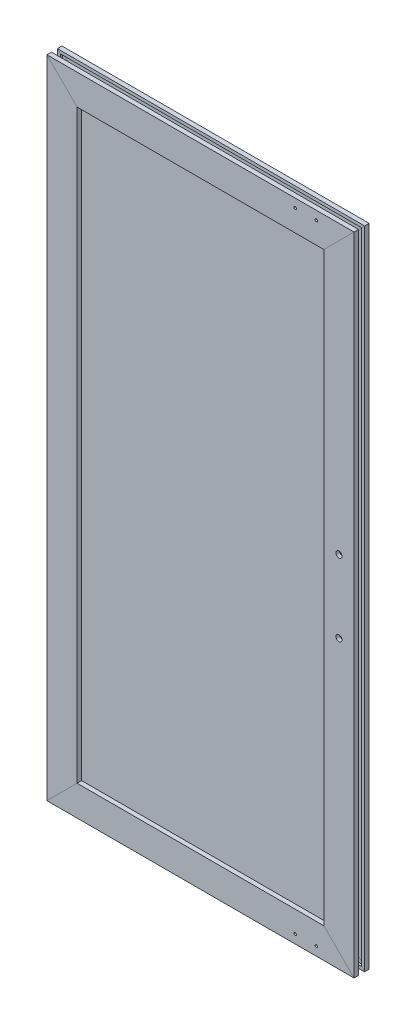
SolidWorks part; units mm, degrees
material "铝型材"
ref_plane "前视基准面" through (0, 0, 0) normal (0, 0, 1) x (1, 0, 0)
ref_plane "上视基准面" through (0, 0, 0) normal (0, 1, 0) x (1, 0, 0)
ref_plane "右视基准面" through (0, 0, 0) normal (1, 0, 0) x (0, 0, -1)
sketch "草图13" plane through (0, 0, 0) normal (0, 0, 1) x (1, 0, 0)
  line L1 (-183.5, -408) -> (183.5, -408)
  line L2 (-183.5, -408) -> (-183.5, 408)
  line L3 (-183.5, 408) -> (183.5, 408)
  line L4 (183.5, -408) -> (183.5, 408)
  line L5 (-183.5, -408) -> (183.5, 408) construction
  line L6 (-183.5, 408) -> (183.5, -408) construction
  point P0 (0, 0)
  dimension "D1" = 367
  dimension "D2" = 816
other "铝型材 2040A(1)"
ref_plane "基准面3" through (-183.5, 408, 0) normal (1, 0, 0) x (0, 1, 0)
sketch "草图19" plane through (-183.5, 408, 0) normal (1, 0, 0) x (0, 1, 0)
  line L0 (9, 4) -> (6, 4)
  line L1 (9, 4) -> (9, 7)
  line L2 (6, -4) -> (6, 4)
  line L3 (16, 7) -> (9, 7)
  line L4 (9, -4) -> (6, -4)
  line L5 (16, 4) -> (16, 7)
  line L6 (9, -7) -> (9, -4)
  line L7 (20, 4) -> (16, 4)
  line L8 (16, -7) -> (9, -7)
  line L9 (20, 10) -> (20, 4)
  line L10 (16, -7) -> (16, -4)
  line L11 (-20, 10) -> (20, 10)
  line L12 (20, -4) -> (16, -4)
  line L13 (-20, 4) -> (-20, 10)
  line L14 (20, -4) -> (20, -10)
  line L15 (-20, 4) -> (-16, 4)
  line L16 (20, -10) -> (-20, -10)
  line L17 (-16, 4) -> (-16, 7)
  line L18 (-20, -10) -> (-20, -4)
  line L19 (-16, 7) -> (-9, 7)
  line L20 (-20, -4) -> (-16, -4)
  line L21 (-9, 4) -> (-9, 7)
  line L22 (-16, -7) -> (-16, -4)
  line L23 (-9, 4) -> (-6, 4)
  line L24 (-16, -7) -> (-9, -7)
  line L25 (-6, -4) -> (-6, 4)
  line L26 (-9, -7) -> (-9, -4)
  line L27 (-9, -4) -> (-6, -4)
  circle A0 centre (0, 0) radius 3.25
  point P0 (0, 0)
sketch "草图14" plane through (0, 0, 0) normal (0, 0, 1) x (1, 0, 0)
  line L0 (189.5, 414) -> (192.5, 417) construction
  line L1 (-177, -401.5) -> (177, -401.5)
  line L2 (-177, -401.5) -> (-177, 401.5)
  line L3 (-177, 401.5) -> (177, 401.5)
  line L4 (177, -401.5) -> (177, 401.5)
  line L5 (-177, -401.5) -> (177, 401.5) construction
  line L6 (-177, 401.5) -> (177, -401.5) construction
  line L8 (163.5, 388) -> (-163.5, 388) construction
  point P0 (0, 0)
  dimension "D1" = 13.5
extrude "凸台-拉伸1" add sketch "草图14" along normal mid plane 4 separate body
hole_wizard "M4 螺纹孔2" positions "草图24" profile "草图25" tap size "M4" standard "GB"
sketch "草图24" plane through (0, 0, 10) normal (0, 0, -1) x (-1, 0, 0)
  line L0 (-153.5, 416.5) -> (-125.5, 416.5) construction
  line L7 (0, 0) -> (81.0682, 0) construction
  line L10 (-203.5, 428) -> (203.5, 428) construction
  line L11 (-203.5, -428) -> (-203.5, 428) construction
  point P0 (-153.5, 416.5)
  point P2 (-125.5, 416.5)
  point P29 (-125.5, -416.5)
  point P30 (-153.5, -416.5)
  dimension "D1" = 28
  dimension "D2" = 11.5
  dimension "D3" = 50
cosmetic thread "孔螺蚊线3"
cosmetic thread "孔螺蚊线4"
cosmetic thread "孔螺蚊线9"
cosmetic thread "孔螺蚊线10"
sketch "草图25" plane through (153.5, 416.5, 10) normal (1, 0, 0) x (0, -1, 0)
  line L0 (0, 0) -> (0, 11.0914)
  line L1 (0, 11.0914) -> (1.65, 10.1)
  line L2 (1.65, 10.1) -> (1.65, 0)
  line L5 (1.65, 0) -> (0, 0)
  line L10 (0, 11.0914) -> (-1.65, 10.1) construction
  line L11 (0, -6.35) -> (0, 107.95) construction
  dimension "螺纹孔钻头直径" = 3.3
  dimension "螺纹孔钻头深度" = 10.1
  dimension "导头角度" = 118
hole_wizard "打孔尺寸(%根据)开槽圆柱头螺钉的类型1" positions "草图26" profile "草图27" counterbore size "M4" standard "GB" end condition through all
sketch "草图26" plane through (0, 0, 10) normal (0, 0, 1) x (1, 0, 0)
  line L0 (0, 0) -> (50000, 0) construction
  line L1 (183.5, 424) -> (183.5, -49576) construction
  line L2 (203.5, 428) -> (163.5, 388) construction
  point P0 (183.5, 48)
  point P2 (183.5, -48)
  point P14 (183.5, 408)
  dimension "D1" = 96
sketch "草图27" plane through (183.5, 48, 10) normal (1, 0, 0) x (0, -1, 0)
  line L0 (0, 0) -> (0, 20)
  line L1 (0, 20) -> (2.25, 20)
  line L3 (2.25, 20) -> (2.25, 4.6)
  line L4 (2.25, 4.6) -> (4, 4.6)
  line L5 (4, 4.6) -> (4, 0)
  line L7 (4, 0) -> (0, 0)
  line L11 (0, -6.35) -> (0, 107.95) construction
  dimension "通孔孔直径" = 4.5
  dimension "通孔孔深度" = 20
  dimension "柱形沉头孔直径" = 8
  dimension "柱形沉头孔深度" = 4.6
hole_wizard "M6 螺纹孔1" positions "草图28" profile "草图29" tap size "M6" standard "GB"
sketch "草图28" plane through (0, 0, -10) normal (0, 0, -1) x (-1, 0, 0)
  line L0 (0, 0) -> (50000, 0) construction
  line L1 (183.5, 424) -> (183.5, -49576) construction
  line L2 (163.5, 388) -> (203.5, 428) construction
  line L3 (-203.5, 428) -> (203.5, 428) construction
  line L4 (183.5, -469.5) -> (183.5, 49530.5) construction
  point P0 (183.5, 368)
  point P2 (183.5, 331)
  point P12 (183.5, 408)
  point P19 (183.5, -368)
  point P20 (183.5, -331)
  dimension "D1" = 60
  dimension "D2" = 37
sketch "草图29" plane through (-183.5, 368, -10) normal (1, 0, 0) x (0, 1, 0)
  line L0 (0, 0) -> (0, 18.5022)
  line L1 (0, 18.5022) -> (2.5, 17)
  line L2 (2.5, 17) -> (2.5, 0)
  line L5 (2.5, 0) -> (0, 0)
  line L10 (0, 18.5022) -> (-2.5, 17) construction
  line L11 (0, -6.35) -> (0, 107.95) construction
  dimension "螺纹孔钻头直径" = 5
  dimension "螺纹孔钻头深度" = 17
  dimension "导头角度" = 118
cosmetic thread "孔螺蚊线5"
cosmetic thread "孔螺蚊线6"
cosmetic thread "孔螺蚊线7"
cosmetic thread "孔螺蚊线8"
